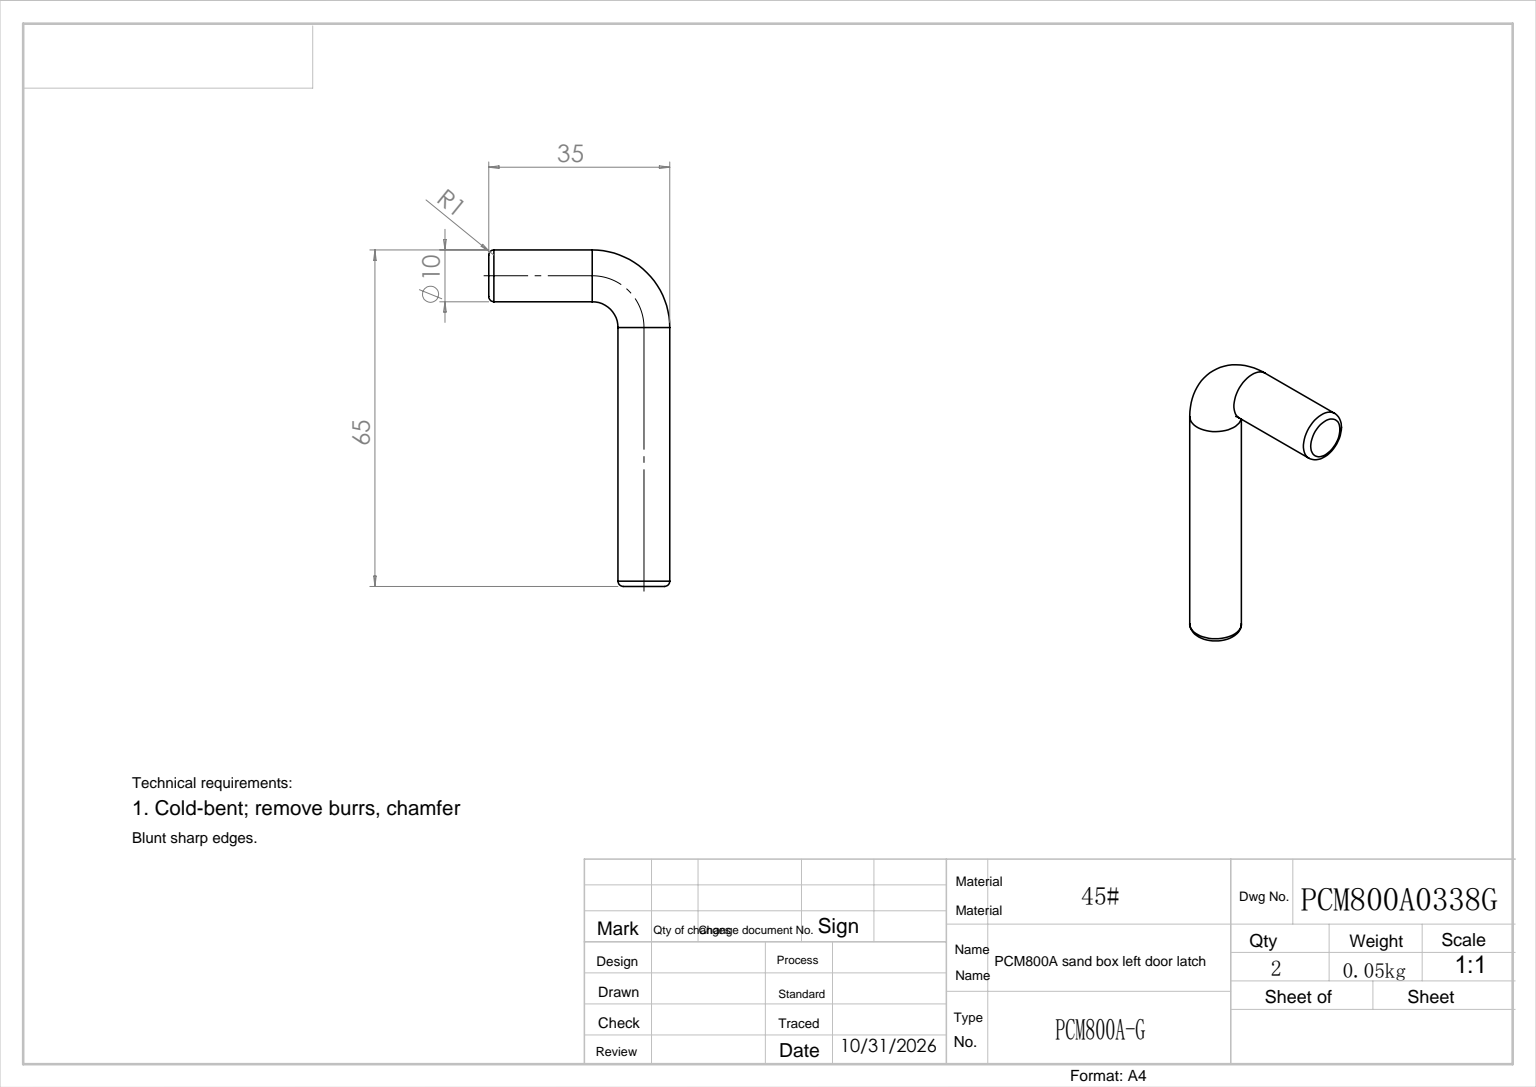
SolidWorks part; units mm, degrees
ref_plane "前视基准面" through (0, 0, 0) normal (0, 0, 1) x (1, 0, 0)
ref_plane "上视基准面" through (0, 0, 0) normal (0, 1, 0) x (1, 0, 0)
ref_plane "右视基准面" through (0, 0, 0) normal (1, 0, 0) x (0, 0, -1)
sketch "草图1" plane through (0, 0, 0) normal (0, 0, 1) x (1, 0, 0)
  line L0 (0, 0) -> (-20, 0)
  line L1 (-30, -10) -> (-30, -60)
  arc A0 (-20, 0) -> (-30, -10) centre (-20, -10) ccw
  point P6 (-30, 0)
  dimension "D3" = 10
  dimension "D1" = 30
  dimension "D2" = 60
sketch "草图2" plane through (0, 0, 0) normal (1, 0, 0) x (0, 0, -1)
  circle A0 centre (0, 0) radius 5
  dimension "D1" = 10
sweep "扫描1" add profiles "草图2" path "草图1"
fillet "圆角1" radius 1 2 edges at (-30, -60, -5) (0, 0, -5)
